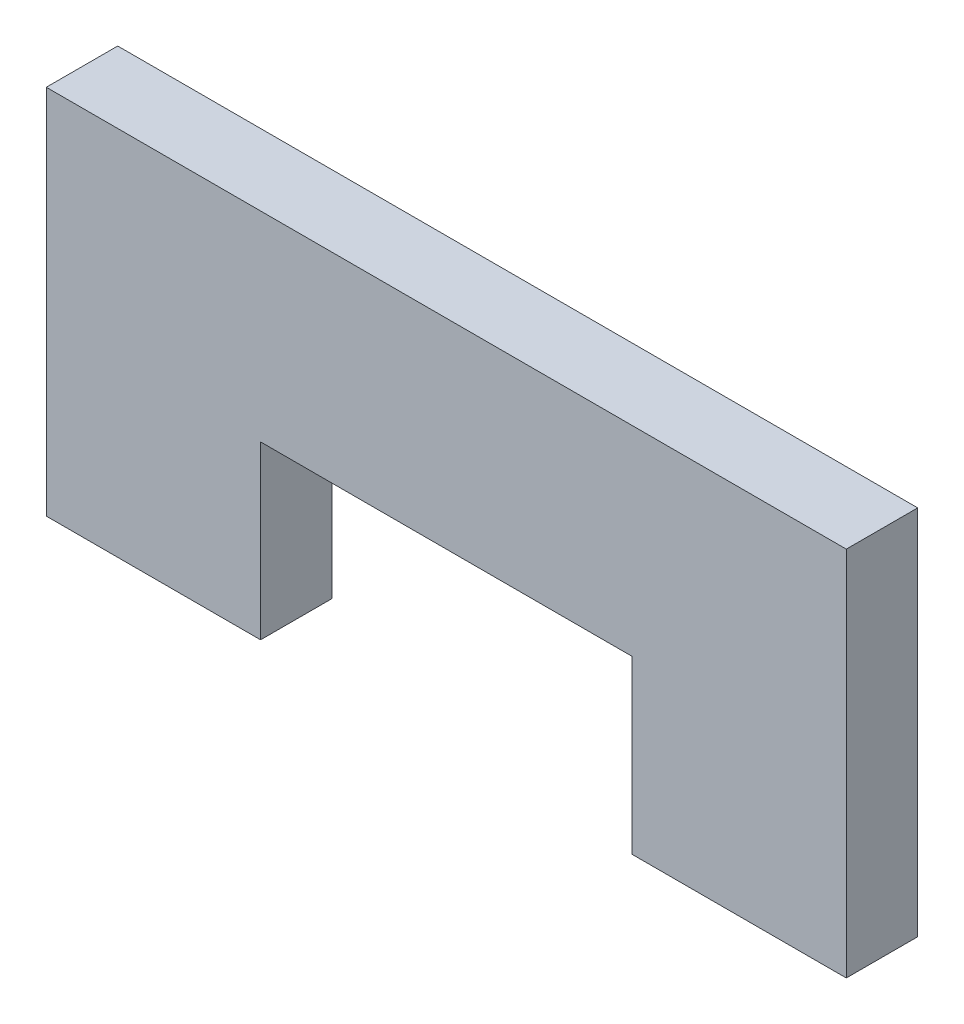
from build123d import *

# Parameters (mm, degrees)
BOSS_EXTRUDE1_DEPTH = 25


with BuildPart() as part:
    # Sketch1 → Boss-Extrude1 (new body)
    with BuildSketch(Plane.XY):
        Polygon((-140, 65), (140, 65), (140, -65), (65, -65), (65, -5), (-65, -5), (-65, -65), (-140, -65), align=None)
    extrude(amount=BOSS_EXTRUDE1_DEPTH)


solid = part.part
